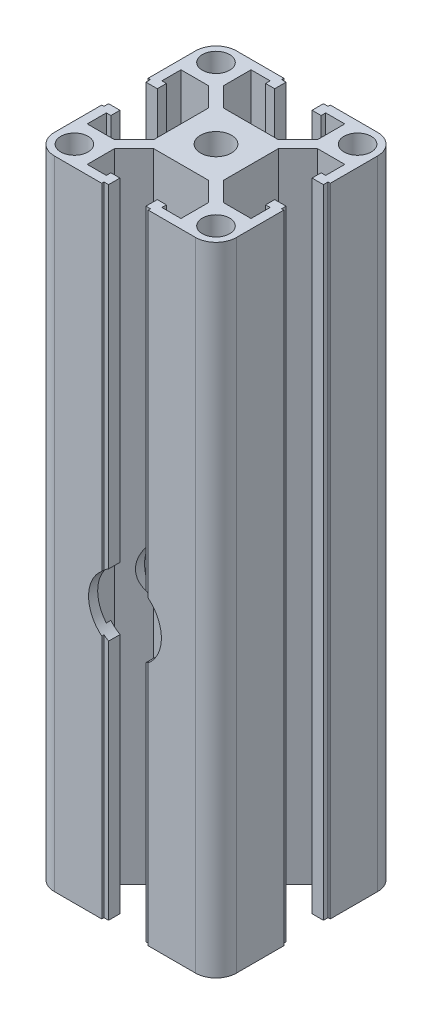
from build123d import *

# Parameters (mm, degrees)
SKETCH16_R                   = 3.4
SKETCH16_R_2                 = 3
MEMBER_1_DEPTH               = 140
HOLE_WIZARD_M8_1_D           = 9
HOLE_WIZARD_M8_1_CBORE_D     = 16
HOLE_WIZARD_M8_1_CBORE_DEPTH = 12.3


with BuildPart() as part:
    # Sketch16 → Member 1 (new body)
    with BuildSketch(Plane(origin=(0, 0, 0), x_dir=(-1, 0, 0), z_dir=(0, 1, 0))):
        with BuildLine():
            Line((-5.1, 20), (-5.1, 19.5))
            Line((-5.1, 19.5), (-4.1, 19.5))
            Line((-4.1, 19.5), (-4.1, 17))
            Line((-4.1, 17), (-6.1, 17))
            Line((-6.1, 17), (-6.1, 18))
            Line((-6.1, 18), (-10.3, 18))
            Line((-10.3, 18), (-10.3, 12))
            Line((-10.3, 12), (-6, 7.7))
            Line((-6, 7.7), (6, 7.7))
            Line((6, 7.7), (10.3, 12))
            Line((10.3, 12), (10.3, 18))
            Line((10.3, 18), (6.1, 18))
            Line((6.1, 18), (6.1, 17))
            Line((6.1, 17), (4.1, 17))
            Line((4.1, 17), (4.1, 19.5))
            Line((4.1, 19.5), (5.1, 19.5))
            Line((5.1, 19.5), (5.1, 20))
            Line((5.1, 20), (15.5, 20))
            ThreePointArc((15.5, 20), (18.681980515, 18.681980515), (20, 15.5))
            Line((20, 15.5), (20, 5.1))
            Line((20, 5.1), (19.5, 5.1))
            Line((19.5, 5.1), (19.5, 4.1))
            Line((19.5, 4.1), (17, 4.1))
            Line((17, 4.1), (17, 6.1))
            Line((17, 6.1), (18, 6.1))
            Line((18, 6.1), (18, 10.3))
            Line((18, 10.3), (12, 10.3))
            Line((12, 10.3), (7.7, 6))
            Line((7.7, 6), (7.7, -6))
            Line((7.7, -6), (12, -10.3))
            Line((12, -10.3), (18, -10.3))
            Line((18, -10.3), (18, -6.1))
            Line((18, -6.1), (17, -6.1))
            Line((17, -6.1), (17, -4.1))
            Line((17, -4.1), (19.5, -4.1))
            Line((19.5, -4.1), (19.5, -5.1))
            Line((19.5, -5.1), (20, -5.1))
            Line((20, -5.1), (20, -15.5))
            ThreePointArc((20, -15.5), (18.681980515, -18.681980515), (15.5, -20))
            Line((15.5, -20), (5.1, -20))
            Line((5.1, -20), (5.1, -19.5))
            Line((5.1, -19.5), (4.1, -19.5))
            Line((4.1, -19.5), (4.1, -17))
            Line((4.1, -17), (6.1, -17))
            Line((6.1, -17), (6.1, -18))
            Line((6.1, -18), (10.3, -18))
            Line((10.3, -18), (10.3, -12))
            Line((10.3, -12), (6, -7.7))
            Line((6, -7.7), (-6, -7.7))
            Line((-6, -7.7), (-10.3, -12))
            Line((-10.3, -12), (-10.3, -18))
            Line((-10.3, -18), (-6.1, -18))
            Line((-6.1, -18), (-6.1, -17))
            Line((-6.1, -17), (-4.1, -17))
            Line((-4.1, -17), (-4.1, -19.5))
            Line((-4.1, -19.5), (-5.1, -19.5))
            Line((-5.1, -19.5), (-5.1, -20))
            Line((-5.1, -20), (-15.5, -20))
            ThreePointArc((-15.5, -20), (-18.681980515, -18.681980515), (-20, -15.5))
            Line((-20, -15.5), (-20, -5.1))
            Line((-20, -5.1), (-19.5, -5.1))
            Line((-19.5, -5.1), (-19.5, -4.1))
            Line((-19.5, -4.1), (-17, -4.1))
            Line((-17, -4.1), (-17, -6.1))
            Line((-17, -6.1), (-18, -6.1))
            Line((-18, -6.1), (-18, -10.3))
            Line((-18, -10.3), (-12, -10.3))
            Line((-12, -10.3), (-7.7, -6))
            Line((-7.7, -6), (-7.7, 6))
            Line((-7.7, 6), (-12, 10.3))
            Line((-12, 10.3), (-18, 10.3))
            Line((-18, 10.3), (-18, 6.1))
            Line((-18, 6.1), (-17, 6.1))
            Line((-17, 6.1), (-17, 4.1))
            Line((-17, 4.1), (-19.5, 4.1))
            Line((-19.5, 4.1), (-19.5, 5.1))
            Line((-19.5, 5.1), (-20, 5.1))
            Line((-20, 5.1), (-20, 15.5))
            ThreePointArc((-20, 15.5), (-18.681980515, 18.681980515), (-15.5, 20))
            Line((-15.5, 20), (-5.1, 20))
        make_face()
        Circle(SKETCH16_R, mode=Mode.SUBTRACT)
        with Locations((-15.556349186, 15.556349186)):
            Circle(SKETCH16_R_2, mode=Mode.SUBTRACT)
        with Locations((15.556349186, 15.556349186)):
            Circle(SKETCH16_R_2, mode=Mode.SUBTRACT)
        with Locations((15.556349186, -15.556349186)):
            Circle(SKETCH16_R_2, mode=Mode.SUBTRACT)
        with Locations((-15.556349186, -15.556349186)):
            Circle(SKETCH16_R_2, mode=Mode.SUBTRACT)
    extrude(amount=MEMBER_1_DEPTH)

    # M8 六角凹头螺钉的柱形沉头孔1 (through all)
    with Locations(Plane(origin=(9.58186976, -44.093066006, 20), x_dir=(-1, 0, 0), z_dir=(0, 0, 1))):
        with Locations((9.58186976, -104.093066006)):
            CounterBoreHole(HOLE_WIZARD_M8_1_D / 2, HOLE_WIZARD_M8_1_CBORE_D / 2, HOLE_WIZARD_M8_1_CBORE_DEPTH)


solid = part.part
